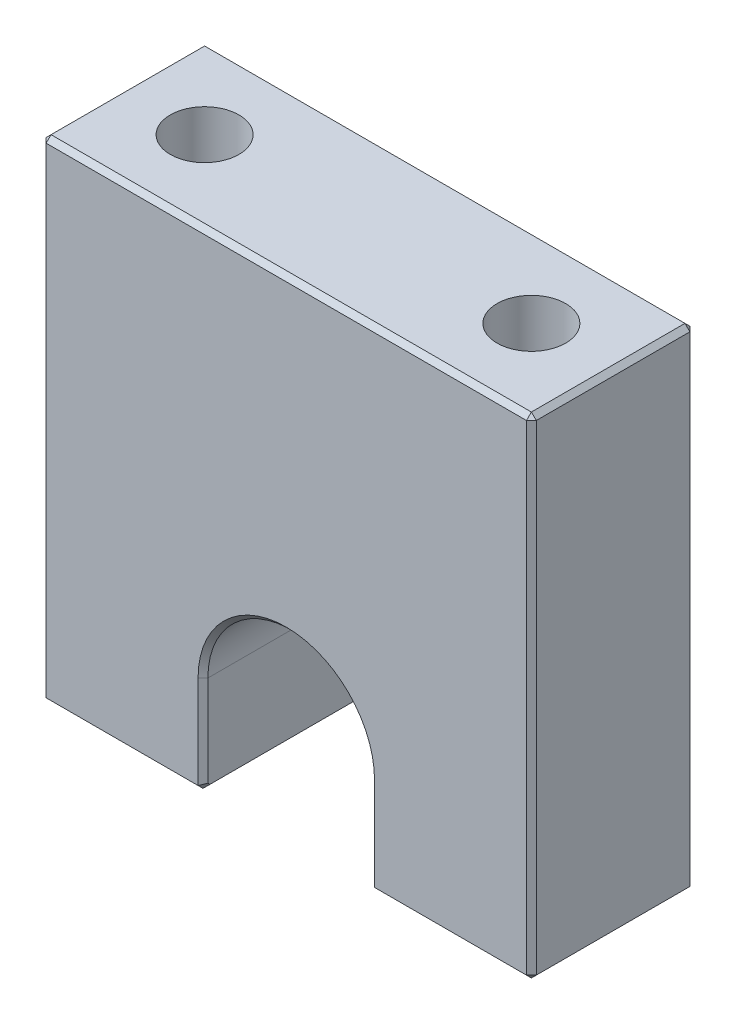
from build123d import *

# Parameters (mm, degrees)
SKETCH_1_W             = 30
SKETCH_1_H             = 30
EXTRUDE_1_DEPTH        = 10
HOLE_WIZARD_M5_1_D     = 4.2
HOLE_WIZARD_M5_1_DEPTH = 16
HOLE_WIZARD_M5_1_TIP   = 1.2618073
CHAMFER_1_SIZE         = 0.3
CUT_EXTRUDE_1_DEPTH    = 24.452078799
CHAMFER_2_SIZE         = 0.3


with BuildPart() as part:
    # 草图1 → 凸台-拉伸1 (new body)
    with BuildSketch(Plane.XY):
        Rectangle(SKETCH_1_W, SKETCH_1_H)
    extrude(amount=EXTRUDE_1_DEPTH)

    # M5 螺纹孔1
    with Locations(Plane(origin=(9.101151333, 15, -0.360612024), x_dir=(-1, 0, 0), z_dir=(0, 1, 0))):
        with Locations((-0.898848667, 5.360612024), (19.101151333, 5.360612024)):
            Hole(HOLE_WIZARD_M5_1_D / 2, depth=HOLE_WIZARD_M5_1_DEPTH)
            with Locations((0, 0, -(HOLE_WIZARD_M5_1_DEPTH + HOLE_WIZARD_M5_1_TIP / 2))):  # 118° drill point
                Cone(0, HOLE_WIZARD_M5_1_D / 2, HOLE_WIZARD_M5_1_TIP, mode=Mode.SUBTRACT)

    # 倒角1
    chamfer_1_edges = [part.edges().sort_by_distance(p)[0] for p in [
        (-15, 0, 10),
        (0, -15, 10),
        (15, 0, 10),
        (0, -15, 0),
        (-15, 0, 0),
        (0, 15, 0),
        (15, 0, 0),
        (0, 15, 10),
        (15, -15, 5),
        (-15, -15, 5),
        (-15, 15, 5),
        (15, 15, 5),
    ]]
    chamfer(chamfer_1_edges, length=CHAMFER_1_SIZE)

    # 草图4 → 切除-拉伸1 (cut, through all)
    with BuildSketch(Plane.XY.offset(10)):
        with BuildLine():
            Line((-5.1, -15), (-5.1, -9))
            ThreePointArc((-5.1, -9), (0, -3.9), (5.1, -9))
            Line((5.1, -9), (5.1, -15))
            ThreePointArc((5.1, -15), (0, -20.1), (-5.1, -15))
        make_face()
    extrude(amount=-CUT_EXTRUDE_1_DEPTH, mode=Mode.SUBTRACT)

    # 倒角2
    chamfer_2_edges = [part.edges().sort_by_distance(p)[0] for p in [
        (5.1, -14.85, 0.15),
        (-5.1, -14.85, 0.15),
        (-5.1, -14.85, 9.85),
        (5.1, -14.85, 9.85),
        (5.1, -15, 5),
        (-5.1, -11.85, 0),
        (-5.1, -15, 5),
        (0, -3.9, 0),
        (5.1, -11.85, 0),
        (5.1, -11.85, 10),
        (0, -3.9, 10),
        (-5.1, -11.85, 10),
    ]]
    chamfer(chamfer_2_edges, length=CHAMFER_2_SIZE)


solid = part.part
